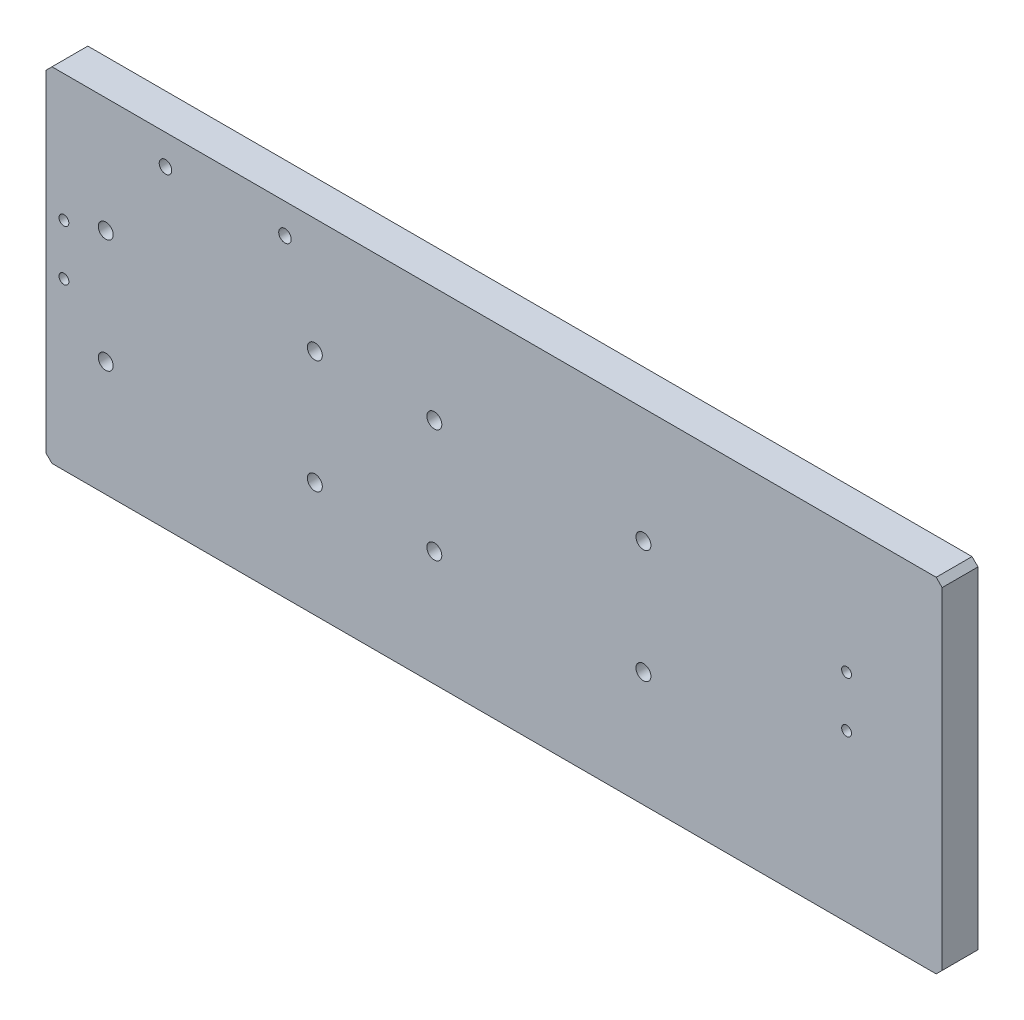
from build123d import *

# Parameters (mm, degrees)
SKETCH_1_W         = 300
SKETCH_1_H         = 115
EXTRUDE_1_DEPTH    = 12
HOLE_WIZARD_M6_1_D = 5
HOLE_WIZARD_M4_2_D = 3.3
HOLE_WIZARD_M5_1_D = 4.2
CHAMFER_1_SIZE     = 2


with BuildPart() as part:
    # 草图1 → 凸台-拉伸1 (new body)
    with BuildSketch(Plane.XY):
        Rectangle(SKETCH_1_W, SKETCH_1_H)
    extrude(amount=EXTRUDE_1_DEPTH)

    # M6 螺纹孔1 (through all)
    with Locations(Plane(origin=(0, 0, 0), x_dir=(-1, 0, 0), z_dir=(0, 0, -1))):
        with Locations((130, 19), (60, -19), (60, 19), (130, -19), (20, 19), (-50, -19), (-50, 19), (20, -19)):
            Hole(HOLE_WIZARD_M6_1_D / 2)

    # M4 螺纹孔2 (through all)
    with Locations(Plane.XY.offset(12)):
        with Locations((-144, 15), (-144, -2), (118, 15), (118, -2)):
            Hole(HOLE_WIZARD_M4_2_D / 2)

    # M5 螺纹孔1 (through all)
    with Locations(Plane(origin=(0, 0, 0), x_dir=(-1, 0, 0), z_dir=(0, 0, -1))):
        with Locations((110, 47.5), (70, 47.5)):
            Hole(HOLE_WIZARD_M5_1_D / 2)

    # 倒角1
    chamfer_1_edges = [part.edges().sort_by_distance(p)[0] for p in [
        (150, -57.5, 6),
        (-150, -57.5, 6),
        (-150, 57.5, 6),
        (150, 57.5, 6),
    ]]
    chamfer(chamfer_1_edges, length=CHAMFER_1_SIZE)


solid = part.part
